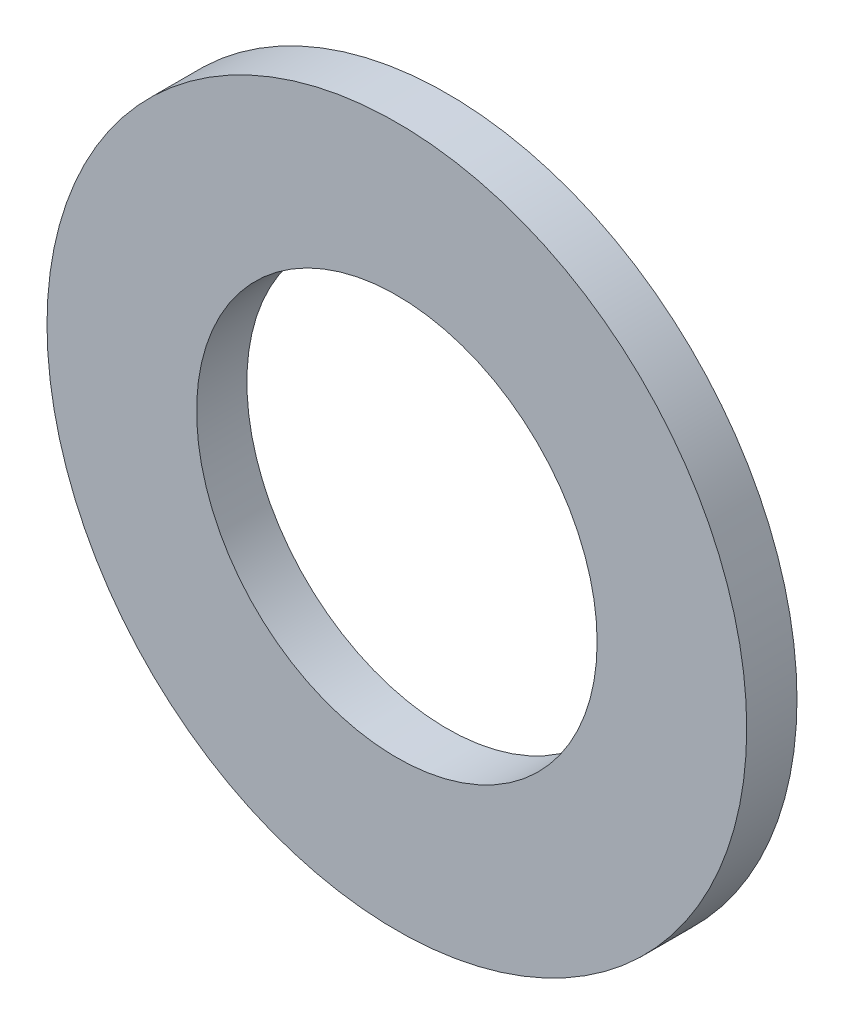
from build123d import *

# Parameters (mm, degrees)
SKETCH1_R           = 11.1379
SKETCH1_R_2         = 6.3754
BOSS_EXTRUDE1_DEPTH = 1.6002


with BuildPart() as part:
    # Sketch1 → Boss-Extrude1 (new body)
    with BuildSketch(Plane.XY):
        Circle(SKETCH1_R)
        Circle(SKETCH1_R_2, mode=Mode.SUBTRACT)
    extrude(amount=BOSS_EXTRUDE1_DEPTH)


solid = part.part
